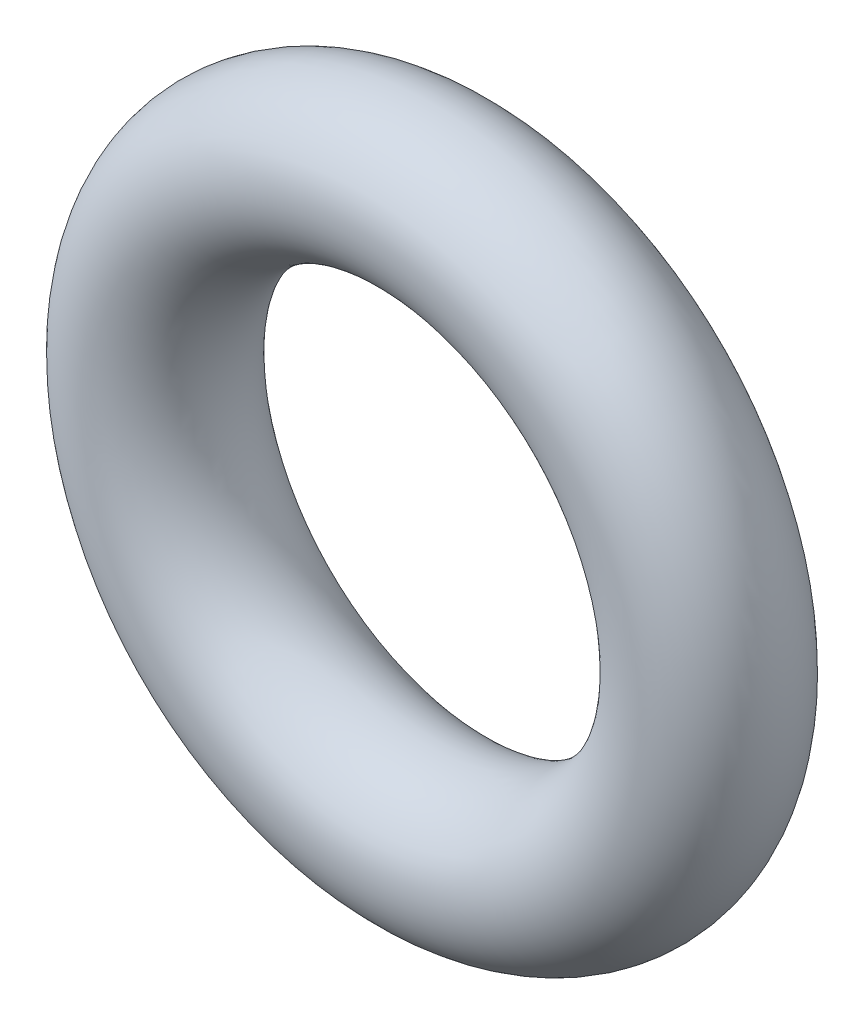
from build123d import *

# Parameters (mm, degrees)
SKETCH1_R = 0.5


with BuildPart() as part:
    # Sketch1 → Revolve1 (revolve)
    with BuildSketch(Plane(origin=(0, 0, 0), x_dir=(1, 0, 0), z_dir=(0, 1, 0))):
        with Locations((-1.8, 0)):
            Circle(SKETCH1_R)
    revolve(axis=Axis((0, 0, 0), (0, 0, 1)))


solid = part.part
